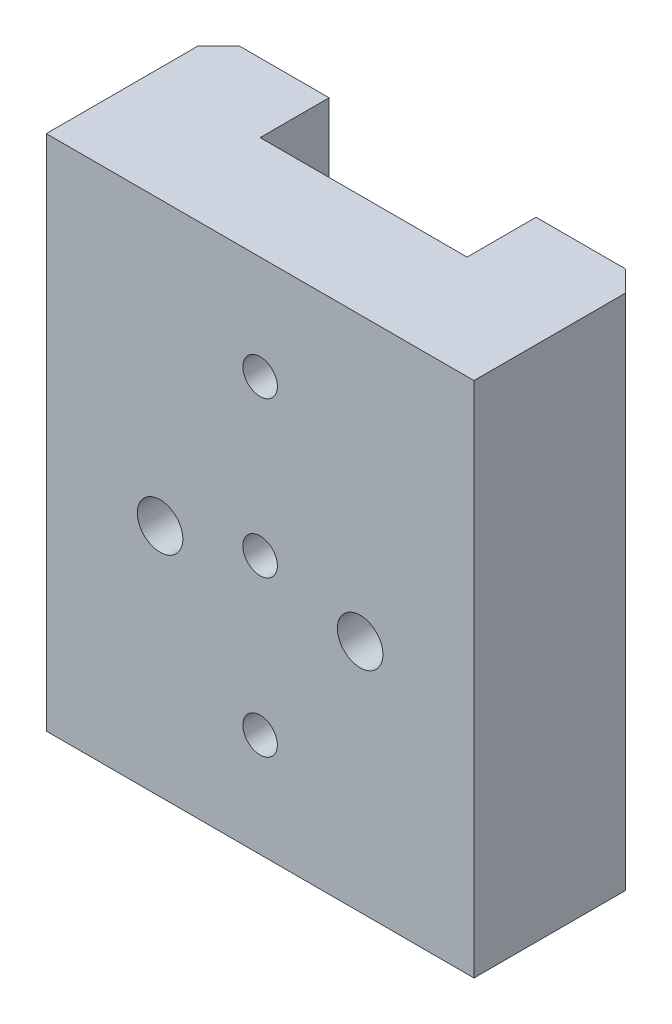
from build123d import *

# Parameters (mm, degrees)
SKETCH_1_W                     = 62
SKETCH_1_H                     = 75
EXTRUDE_1_DEPTH                = 12.5
HOLE_WIZARD_M6_1_D             = 5
CHAMFER_1_SIZE                 = 3
SKETCH_8_W                     = 30
SKETCH_8_H                     = 75
CUT_EXTRUDE_1_DEPTH            = 10
HOLE_WIZARD_M6_2_D             = 5
HOLE_WIZARD_M6_1_2_D           = 6.6
HOLE_WIZARD_M6_1_2_CBORE_D     = 11
HOLE_WIZARD_M6_1_2_CBORE_DEPTH = 20


with BuildPart() as part:
    # 草图1 → 凸台-拉伸1 (new, symmetric)
    with BuildSketch(Plane.XY):
        Rectangle(SKETCH_1_W, SKETCH_1_H)
    extrude(amount=EXTRUDE_1_DEPTH, both=True)

    # Hole Wizard M6 _1 (through all)
    with Locations(Plane.XY.offset(12.5)):
        with Locations((0, 0)):
            Hole(HOLE_WIZARD_M6_1_D / 2)

    # 倒角1
    chamfer_1_edges = [part.edges().sort_by_distance(p)[0] for p in [
        (-31, 0, -12.5),
        (31, 0, -12.5),
    ]]
    chamfer(chamfer_1_edges, length=CHAMFER_1_SIZE)

    # 草图8 → 切除-拉伸1 (cut)
    with BuildSketch(Plane(origin=(0, 0, -12.5), x_dir=(-1, 0, 0), z_dir=(0, 0, -1))):
        Rectangle(SKETCH_8_W, SKETCH_8_H)
    extrude(amount=-CUT_EXTRUDE_1_DEPTH, mode=Mode.SUBTRACT)

    # M6 螺纹孔2 (through all)
    with Locations(Plane(origin=(0, 0, -2.5), x_dir=(-1, 0, 0), z_dir=(0, 0, -1))):
        with Locations((0, 22.5), (0, -22.5)):
            Hole(HOLE_WIZARD_M6_2_D / 2)

    # Hole Wizard M6 _1 2 (through all)
    with Locations(Plane(origin=(0, 0, -12.5), x_dir=(-1, 0, 0), z_dir=(0, 0, -1))):
        with Locations((-14.5, -3.5), (14.5, -3.5)):
            CounterBoreHole(HOLE_WIZARD_M6_1_2_D / 2, HOLE_WIZARD_M6_1_2_CBORE_D / 2, HOLE_WIZARD_M6_1_2_CBORE_DEPTH)


solid = part.part
